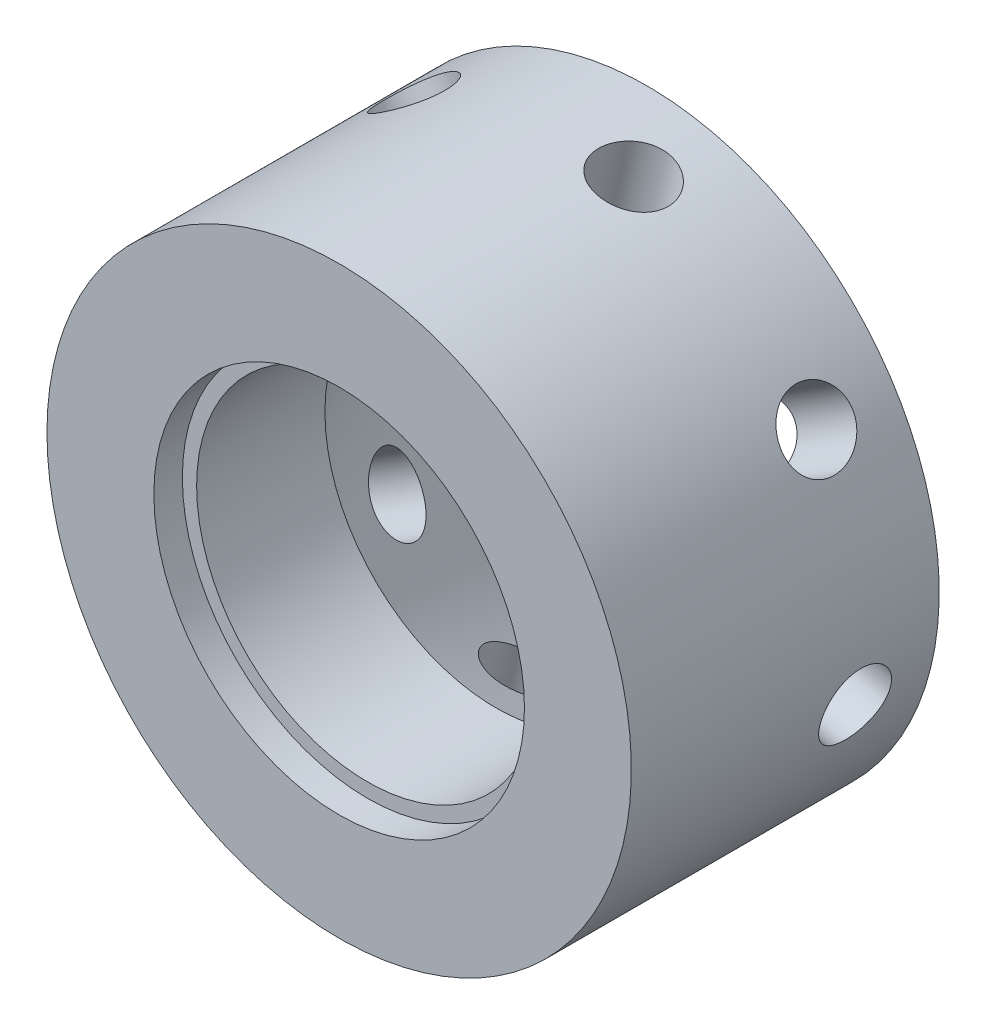
SolidWorks part; units mm, degrees
ref_plane "Front Plane" through (0, 0, 0) normal (0, 0, 1) x (1, 0, 0)
ref_plane "Top Plane" through (0, 0, 0) normal (0, 1, 0) x (1, 0, 0)
ref_plane "Right Plane" through (0, 0, 0) normal (1, 0, 0) x (0, 0, -1)
ref_plane "Plane1" through (0, 234.744, 0) normal (0, -1, 0) x (1, 0, 0)
sketch "Sketch1" plane through (0, 234.744, 0) normal (0, -1, 0) x (1, 0, 0)
  line L0 (623.7306, -1044.693) -> (521.2306, -1044.693)
  line L1 (521.2306, -1044.693) -> (521.2306, -1152.693)
  line L2 (521.2306, -1152.693) -> (623.7306, -1152.693)
  line L3 (623.7306, -1152.693) -> (623.7306, -1044.693)
  line L4 (521.2306, -1044.693) -> (521.2306, -1152.693) construction
  dimension "D1" = 102.5
  dimension "D2" = 108
revolve "Revolve1" add sketch "Sketch1" angle 360 about L4
ref_plane "Plane2" through (0, 234.744, 0) normal (0, 1, 0) x (1, 0, 0)
sketch "Sketch2" plane through (0, 234.744, 0) normal (0, 1, 0) x (1, 0, 0)
  line L0 (606.2306, 1152.693) -> (521.2306, 1152.693)
  line L1 (521.2306, 1152.693) -> (521.2306, 1044.693)
  line L2 (521.2306, 1044.693) -> (586.2306, 1044.693)
  line L3 (586.2306, 1044.693) -> (586.2306, 1054.693)
  line L4 (586.2306, 1054.693) -> (581.2306, 1054.693)
  line L5 (581.2306, 1054.693) -> (581.2306, 1099.693)
  line L6 (581.2306, 1099.693) -> (606.2306, 1152.693)
  line L7 (521.2306, 1152.693) -> (521.2306, 1044.693) construction
  dimension "D1" = 60
  dimension "D2" = 65
  dimension "D3" = 85
  dimension "D4" = 10
  dimension "D5" = 55
  dimension "D6" = 108
revolve "Cut-Revolve1" cut sketch "Sketch2" angle 360 about L7
hole_wizard "Ø25.0 (25) diameter hole1" positions "3D sketch1" profile "Sketch3" hole size "Ø25.0" standard "ANSI Metric"
sketch3d "3D sketch1"
  point P0 (434.6759, 179.8393, -1125.693)
sketch "Sketch3" plane through (434.6759, 179.8393, -1125.693) normal (0, 0, 1) x (0.5357, -0.8444, 0)
  line L0 (0, 0) -> (0, 30.2358)
  line L1 (0, 30.2358) -> (12.5, 30.2358)
  line L2 (12.5, 30.2358) -> (12.5, 0)
  line L5 (12.5, 0) -> (0, 0)
  line L11 (0, -6.35) -> (0, 107.95) construction
  dimension "通孔孔直径" = 25
  dimension "通孔孔深度" = 30.2358
hole_wizard "Ø25.0 (25) diameter hole2" positions "3D sketch2" profile "Sketch4" hole size "Ø25.0" standard "ANSI Metric"
sketch3d "3D sketch2"
  point P0 (421.2037, 257.124, -1125.693)
sketch "Sketch4" plane through (421.2037, 257.124, -1125.693) normal (0, 0, 1) x (-0.2183, -0.9759, 0)
  line L0 (0, 0) -> (0, 30.2358)
  line L1 (0, 30.2358) -> (12.5, 30.2358)
  line L2 (12.5, 30.2358) -> (12.5, 0)
  line L5 (12.5, 0) -> (0, 0)
  line L11 (0, -6.35) -> (0, 107.95) construction
  dimension "通孔孔直径" = 25
  dimension "通孔孔深度" = 30.2358
hole_wizard "Ø25.0 (25) diameter hole3" positions "3D sketch3" profile "Sketch5" hole size "Ø25.0" standard "ANSI Metric"
sketch3d "3D sketch3"
  point P0 (466.326, 321.2987, -1125.693)
sketch "Sketch5" plane through (466.326, 321.2987, -1125.693) normal (0, 0, 1) x (-0.8444, -0.5357, 0)
  line L0 (0, 0) -> (0, 30.2358)
  line L1 (0, 30.2358) -> (12.5, 30.2358)
  line L2 (12.5, 30.2358) -> (12.5, 0)
  line L5 (12.5, 0) -> (0, 0)
  line L11 (0, -6.35) -> (0, 107.95) construction
  dimension "通孔孔直径" = 25
  dimension "通孔孔深度" = 30.2358
hole_wizard "Ø25.0 (25) diameter hole4" positions "3D sketch4" profile "Sketch6" hole size "Ø25.0" standard "ANSI Metric"
sketch3d "3D sketch4"
  point P0 (543.6107, 334.7709, -1125.693)
sketch "Sketch6" plane through (543.6107, 334.7709, -1125.693) normal (0, 0, 1) x (-0.9759, 0.2183, 0)
  line L0 (0, 0) -> (0, 30.2358)
  line L1 (0, 30.2358) -> (12.5, 30.2358)
  line L2 (12.5, 30.2358) -> (12.5, 0)
  line L5 (12.5, 0) -> (0, 0)
  line L11 (0, -6.35) -> (0, 107.95) construction
  dimension "通孔孔直径" = 25
  dimension "通孔孔深度" = 30.2358
hole_wizard "Ø25.0 (25) diameter hole5" positions "3D sketch5" profile "Sketch7" hole size "Ø25.0" standard "ANSI Metric"
sketch3d "3D sketch5"
  point P0 (607.7854, 289.6486, -1125.693)
sketch "Sketch7" plane through (607.7854, 289.6486, -1125.693) normal (0, 0, 1) x (-0.5357, 0.8444, 0)
  line L0 (0, 0) -> (0, 243.9594)
  line L1 (0, 243.9594) -> (12.5, 243.9594)
  line L2 (12.5, 243.9594) -> (12.5, 0)
  line L5 (12.5, 0) -> (0, 0)
  line L11 (0, -6.35) -> (0, 107.95) construction
  dimension "通孔孔直径" = 25
  dimension "通孔孔深度" = 243.9594
hole_wizard "Ø25.0 (25) diameter hole6" positions "3D sketch6" profile "Sketch8" hole size "Ø25.0" standard "ANSI Metric"
sketch3d "3D sketch6"
  point P0 (621.2576, 212.3639, -1125.693)
sketch "Sketch8" plane through (621.2576, 212.3639, -1125.693) normal (0, 0, 1) x (0.2183, 0.9759, 0)
  line L0 (0, 0) -> (0, 224.9069)
  line L1 (0, 224.9069) -> (12.5, 224.9069)
  line L2 (12.5, 224.9069) -> (12.5, 0)
  line L5 (12.5, 0) -> (0, 0)
  line L11 (0, -6.35) -> (0, 107.95) construction
  dimension "通孔孔直径" = 25
  dimension "通孔孔深度" = 224.9069
hole_wizard "Ø25.0 (25) diameter hole7" positions "3D sketch7" profile "Sketch9" hole size "Ø25.0" standard "ANSI Metric"
sketch3d "3D sketch7"
  point P0 (576.1353, 148.1892, -1125.693)
sketch "Sketch9" plane through (576.1353, 148.1892, -1125.693) normal (0, 0, 1) x (0.8444, 0.5357, 0)
  line L0 (0, 0) -> (0, 243.9594)
  line L1 (0, 243.9594) -> (12.5, 243.9594)
  line L2 (12.5, 243.9594) -> (12.5, 0)
  line L5 (12.5, 0) -> (0, 0)
  line L11 (0, -6.35) -> (0, 107.95) construction
  dimension "通孔孔直径" = 25
  dimension "通孔孔深度" = 243.9594
hole_wizard "Ø25.0 (25) diameter hole8" positions "3D sketch8" profile "Sketch10" hole size "Ø25.0" standard "ANSI Metric"
sketch3d "3D sketch8"
  point P0 (498.8506, 134.717, -1125.693)
sketch "Sketch10" plane through (498.8506, 134.717, -1125.693) normal (0, 0, 1) x (0.9759, -0.2183, 0)
  line L0 (0, 0) -> (0, 224.9069)
  line L1 (0, 224.9069) -> (12.5, 224.9069)
  line L2 (12.5, 224.9069) -> (12.5, 0)
  line L5 (12.5, 0) -> (0, 0)
  line L11 (0, -6.35) -> (0, 107.95) construction
  dimension "通孔孔直径" = 25
  dimension "通孔孔深度" = 224.9069
